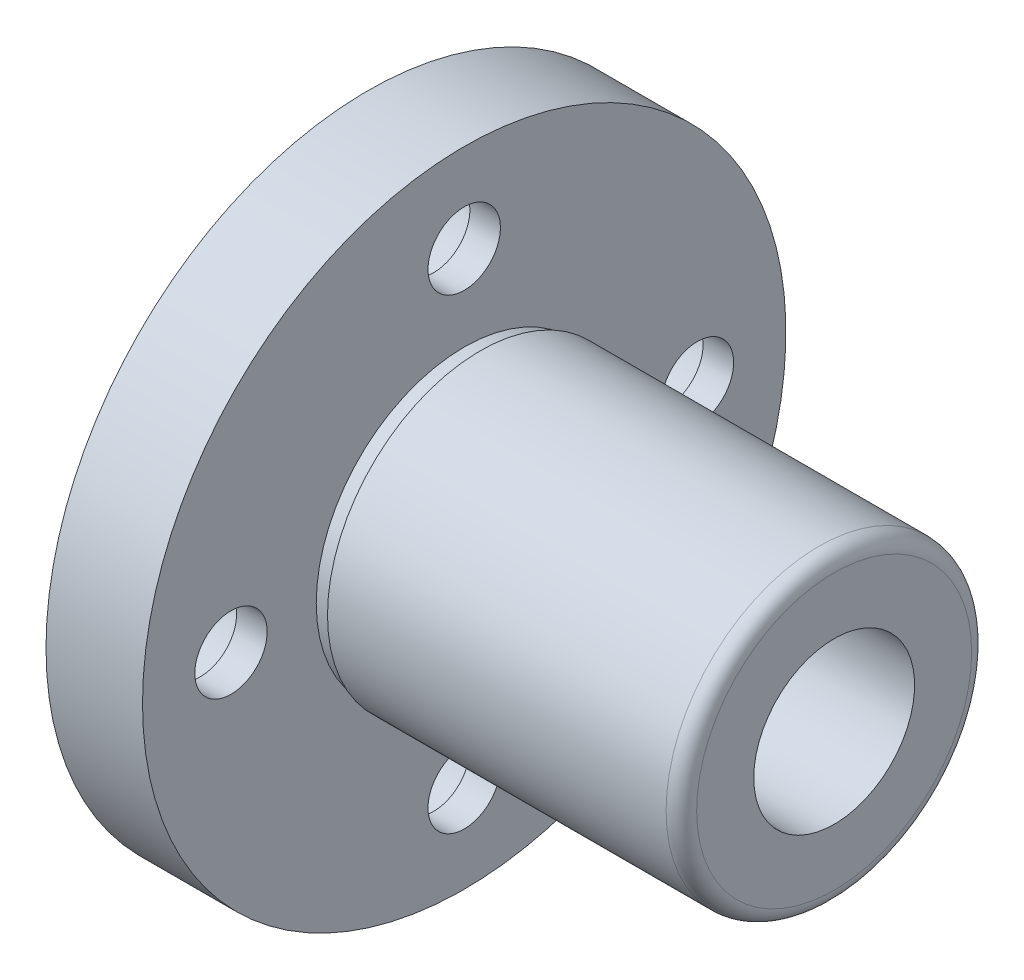
from build123d import *

# Parameters (mm, degrees)
PATTERN_LINEAR_1_COUNT      = 2
PATTERN_LINEAR_1_PITCH      = 20.506096654
PATTERN_LINEAR_1_COUNT_DIR2 = 2
PATTERN_LINEAR_1_PITCH_DIR2 = 20.506096654


with BuildPart() as part:
    # 草图1 → 旋转1 (revolve)
    with BuildSketch(Plane.XY, mode=Mode.PRIVATE) as revolve_1_sk:
        with BuildLine():
            Line((0, 20), (0, 5))
            Line((0, 5), (29, 5))
            Line((29, 5), (29, 8.55))
            ThreePointArc((29, 8.55), (28.721751442, 9.221751442), (28.05, 9.5))
            Line((28.05, 9.5), (7, 9.5))
            Line((7, 9.5), (7, 9.2))
            Line((7, 9.2), (6, 9.2))
            Line((6, 9.2), (6, 20))
            Line((6, 20), (0, 20))
        make_face()
    revolve(revolve_1_sk.sketch.rotate(Axis((29, 0, 0), (-1, 0, 0)), 270), axis=Axis((29, 0, 0), (-1, 0, 0)))

    # 草图2 → 切除-旋转1 (revolve, cut)
    with BuildSketch(Plane.XY, mode=Mode.PRIVATE) as cut_revolve_1_sk:
        Polygon((0, 14.5), (0, 18.25), (4.1, 18.25), (4.1, 16.75), (6, 16.75), (6, 14.5), align=None)
    cut_revolve_1 = revolve(cut_revolve_1_sk.sketch.rotate(Axis((6, 14.5, 0), (-1, 0, 0)), 270), axis=Axis((6, 14.5, 0), (-1, 0, 0)), mode=Mode.SUBTRACT)

    # 阵列(线性)1: Cut-Revolve 1 2 × 2
    with Locations(*[Vector(0, -0.7071067811865475, 0.7071067811865477) * (i * PATTERN_LINEAR_1_PITCH) + Vector(0, -0.7071067811865477, -0.7071067811865474) * (j * PATTERN_LINEAR_1_PITCH_DIR2) for i in range(PATTERN_LINEAR_1_COUNT) for j in range(PATTERN_LINEAR_1_COUNT_DIR2) if (i, j) != (0, 0)]):
        add(cut_revolve_1, mode=Mode.SUBTRACT)


solid = part.part
